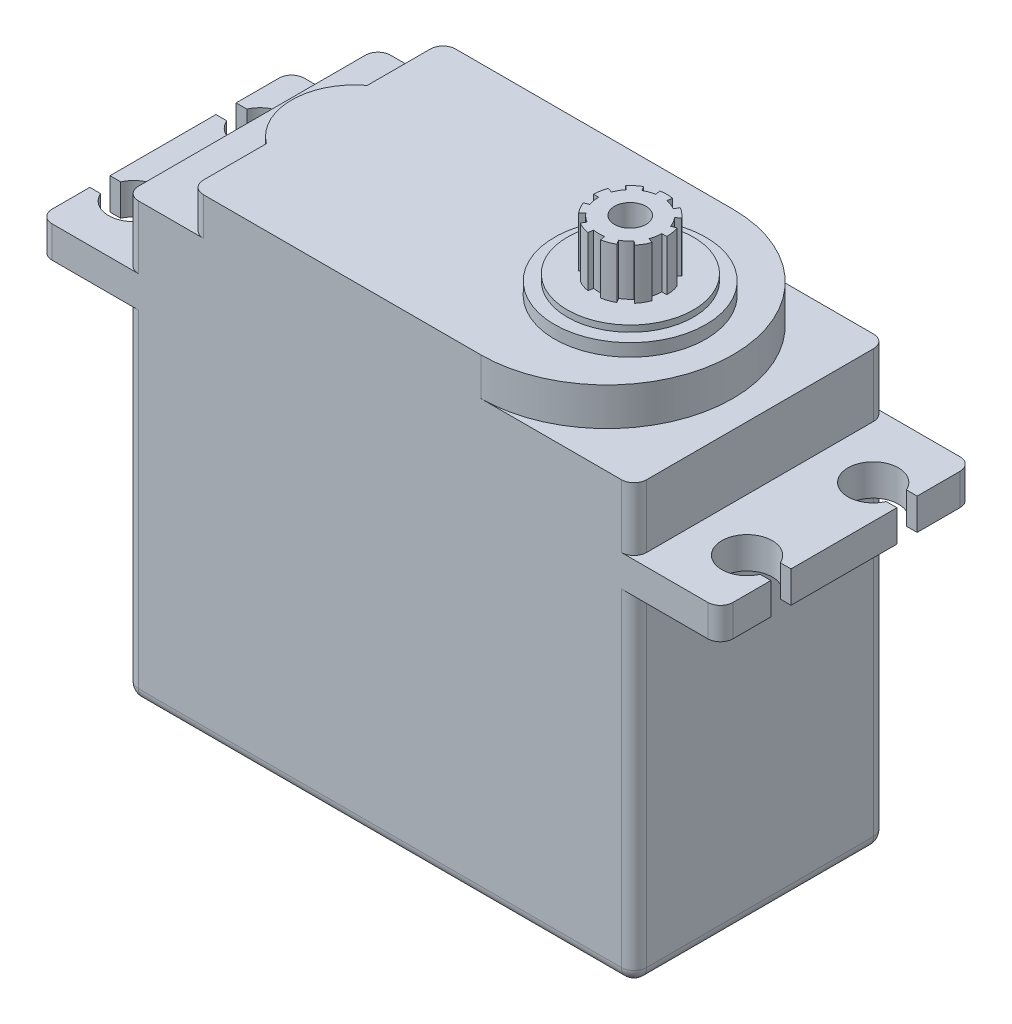
SolidWorks part; units mm, degrees
ref_plane "前视基准面" through (0, 0, 0) normal (0, 0, 1) x (1, 0, 0)
ref_plane "上视基准面" through (0, 0, 0) normal (0, 1, 0) x (1, 0, 0)
ref_plane "右视基准面" through (0, 0, 0) normal (1, 0, 0) x (0, 0, -1)
sketch "草图1" plane through (0, 0, 0) normal (0, 0, 1) x (1, 0, 0)
  line L0 (0, 0) -> (-50000, 0) construction
  line L1 (0, 0) -> (0, 50000) construction
  line L2 (20.15, 8) -> (27, 8)
  line L3 (-20.15, 18.5) -> (20.15, 18.5)
  line L4 (-20.15, 18.5) -> (-20.15, 10.5)
  line L5 (-20.15, -19) -> (20.15, -19)
  line L6 (20.15, 18.5) -> (20.15, 10.5)
  line L7 (-27, 10.5) -> (-20.15, 10.5)
  line L8 (-27, 10.5) -> (-27, 8)
  line L9 (-27, 8) -> (-20.15, 8)
  line L10 (27, 10.5) -> (27, 8)
  line L11 (20.15, 10.5) -> (27, 10.5)
  line L12 (20.15, 8) -> (20.15, -19)
  line L13 (-20.15, 8) -> (-20.15, -19)
  dimension "D1" = 8
  dimension "D2" = 6.85
  dimension "D3" = 2.5
  dimension "D4" = 40.3
  dimension "D5" = 27
  dimension "D6" = 54
  dimension "D7" = 20.15
extrude "凸台-拉伸1" add sketch "草图1" along normal blind 20
fillet "圆角1" radius 1 18 edges at (-20.15, 14.5, 20) (20.15, 14.5, 20) (20.15, 18.5, 10) (-20.15, 18.5, 10) (20.15, 14.5, 0) (-20.15, 14.5, 0) (-20.15, -19, 10) (0, -19, 20) (20.15, -19, 10) (0, -19, 0) (-20.15, -5.5, 0) (20.15, -5.5, 0) (20.15, -5.5, 20) (-20.15, -5.5, 20) (27, 9.25, 0) (27, 9.25, 20) (-27, 9.25, 0) (-27, 9.25, 20)
sketch "草图2" plane through (0, 10.5, 0) normal (0, 1, 0) x (1, 0, 0)
  line L0 (-0.1717, -10.2) -> (49999.8283, -10.2) construction
  line L1 (0, 0) -> (0, -50000) construction
  line L2 (-26.148, -4.4) -> (-29.2227, -4.4)
  line L3 (-24.315, -5.2) -> (-30.8838, -5.2) construction
  line L4 (-24, -15) -> (-30.5688, -15) construction
  line L5 (-29.2227, -4.4) -> (-29.2227, -6)
  line L6 (-26.148, -6) -> (-29.2227, -6)
  line L7 (-26.148, -14.4) -> (-29.2227, -14.4)
  line L8 (-29.2227, -16) -> (-29.2227, -14.4)
  line L9 (-26.148, -16) -> (-29.2227, -16)
  line L10 (26.148, -16) -> (29.2227, -16)
  line L11 (29.2227, -16) -> (29.2227, -14.4)
  line L12 (26.148, -14.4) -> (29.2227, -14.4)
  line L13 (29.2227, -4.4) -> (29.2227, -6)
  line L14 (26.148, -6) -> (29.2227, -6)
  line L15 (26.148, -4.4) -> (29.2227, -4.4)
  arc A0 (-26.148, -14.4) -> (-26.148, -16) centre (-24.315, -15.2) cw
  arc A1 (26.148, -14.4) -> (26.148, -16) centre (24.315, -15.2) ccw
  arc A2 (-26.148, -6) -> (-26.148, -4.4) centre (-24.315, -5.2) ccw
  arc A3 (26.148, -6) -> (26.148, -4.4) centre (24.315, -5.2) cw
  point P21 (-29.2227, -5.2)
  dimension "D2" = 10
  dimension "D1" = 48.63
  dimension "D3" = 2
extrude "切除-拉伸1" cut sketch "草图2" against normal blind 20
sketch "草图3" plane through (0, 18.5, 0) normal (0, 1, 0) x (1, 0, 0)
  line L0 (-40.2617, -10) -> (49959.7383, -10) construction
  line L1 (-14, 0) -> (8, 0)
  line L2 (-15, -1) -> (-15, -6)
  line L3 (-14, -20) -> (8, -20)
  line L4 (-15, -14) -> (-15, -19)
  line L5 (0, 0) -> (0, 50000) construction
  line L7 (-26.8677, 6.7729) -> (25, 6.7729)
  line L8 (-26.8677, 6.7729) -> (-26.8677, -28.4888)
  line L9 (-26.8677, -28.4888) -> (25, -28.4888)
  line L10 (25, 6.7729) -> (25, -28.4888)
  arc A0 (8, -20) -> (8, 0) centre (8, -10) ccw
  arc A1 (-15, -6) -> (-15, -14) centre (-12, -10) ccw
  arc A2 (-14, -20) -> (-15, -19) centre (-14, -19) cw
  arc A3 (-15, -1) -> (-14, 0) centre (-14, -1) cw
  dimension "D2" = 1
  dimension "D1" = 25
extrude "切除-拉伸2" cut sketch "草图3" against normal blind 3
sketch "草图4" plane through (0, 18.5, 0) normal (0, 1, 0) x (1, 0, 0)
  line L0 (27, -14.4) -> (27, -6) construction
  circle A0 centre (9.85, -10) radius 6
  dimension "D1" = 17.15
extrude "凸台-拉伸2" add sketch "草图4" along normal blind 1
sketch "草图5" plane through (0, 19.5, 0) normal (0, 1, 0) x (1, 0, 0)
  line L0 (27, -14.4) -> (27, -6) construction
  circle A0 centre (9.8513, -9.9876) radius 5
  point P2 (27, -10.2)
  dimension "D1" = 17.15
extrude "凸台-拉伸3" add sketch "草图5" along normal blind 0.5
sketch "草图6" plane through (0, 20, 0) normal (0, 1, 0) x (1, 0, 0)
  line L1 (10.2841, -7.538) -> (10.3536, -7.1441)
  line L3 (11.3, -7.4885) -> (11.1, -7.8349)
  line L5 (12.0715, -8.1359) -> (11.7651, -8.393)
  line L7 (12.5751, -9.0081) -> (12.1992, -9.1449)
  line L8 (6.95, -10) -> (7.35, -10)
  line L10 (7.5008, -9.1449) -> (7.1249, -9.0081)
  line L13 (8.6, -7.8349) -> (8.4, -7.4885)
  line L14 (7.9349, -8.393) -> (7.6285, -8.1359)
  line L15 (9.4159, -7.538) -> (9.3464, -7.1441)
  line L16 (9.4159, -12.462) -> (9.3464, -12.8559)
  line L19 (8.4, -12.5115) -> (8.6, -12.1651)
  line L20 (27, -14.4) -> (27, -6) construction
  line L21 (7.6285, -11.8641) -> (7.9349, -11.607)
  line L23 (7.1249, -10.9919) -> (7.5008, -10.8551)
  line L25 (12.1992, -10.8551) -> (12.5751, -10.9919)
  line L28 (11.1, -12.1651) -> (11.3, -12.5115)
  line L29 (10.2841, -12.462) -> (10.3536, -12.8559)
  line L30 (11.7651, -11.607) -> (12.0715, -11.8641)
  line L31 (12.35, -10) -> (12.75, -10)
  arc A0 (7.1249, -10.9919) -> (7.6285, -11.8641) centre (9.85, -10) ccw
  arc A1 (7.35, -10) -> (7.5008, -10.8551) centre (9.85, -10) ccw
  arc A2 (7.1249, -9.0081) -> (6.95, -10) centre (9.85, -10) ccw
  arc A3 (8.4, -7.4885) -> (7.6285, -8.1359) centre (9.85, -10) ccw
  arc A4 (10.3536, -7.1441) -> (9.3464, -7.1441) centre (9.85, -10) ccw
  arc A5 (12.0715, -8.1359) -> (11.3, -7.4885) centre (9.85, -10) ccw
  arc A6 (12.75, -10) -> (12.5751, -9.0081) centre (9.85, -10) ccw
  arc A7 (12.0715, -11.8641) -> (12.5751, -10.9919) centre (9.85, -10) ccw
  arc A8 (10.3536, -12.8559) -> (11.3, -12.5115) centre (9.85, -10) ccw
  arc A9 (8.4, -12.5115) -> (9.3464, -12.8559) centre (9.85, -10) ccw
  arc A10 (7.9349, -8.393) -> (7.5008, -9.1449) centre (9.85, -10) ccw
  arc A11 (9.4159, -7.538) -> (8.6, -7.8349) centre (9.85, -10) ccw
  arc A12 (11.1, -7.8349) -> (10.2841, -7.538) centre (9.85, -10) ccw
  arc A13 (12.1992, -9.1449) -> (11.7651, -8.393) centre (9.85, -10) ccw
  arc A14 (12.1992, -10.8551) -> (12.35, -10) centre (9.85, -10) ccw
  arc A15 (11.1, -12.1651) -> (11.7651, -11.607) centre (9.85, -10) ccw
  arc A16 (9.4159, -12.462) -> (10.2841, -12.462) centre (9.85, -10) ccw
  arc A17 (7.9349, -11.607) -> (8.6, -12.1651) centre (9.85, -10) ccw
  circle A18 centre (9.85, -10) radius 1
  dimension "D1" = 17.15
extrude "凸台-拉伸4" add sketch "草图6" along normal blind 4
hole_wizard "M3 螺纹孔1" positions "3D草图2" profile "草图8" tap size "M3" standard "GB"
sketch3d "3D草图2"
  line L0 (9.85, 24, 10) -> (9.85, 20, 10) construction
  point P0 (9.85, 24, 10)
sketch "草图8" plane through (9.85, 24, 10) normal (1, 0, 0) x (0, 0, 1)
  line L0 (0, 0) -> (0, 8.2511)
  line L1 (0, 8.2511) -> (1.25, 7.5)
  line L2 (1.25, 7.5) -> (1.25, 0)
  line L5 (1.25, 0) -> (0, 0)
  line L10 (0, 8.2511) -> (-1.25, 7.5) construction
  line L11 (0, -6.35) -> (0, 107.95) construction
  dimension "螺纹孔钻头直径" = 2.5
  dimension "螺纹孔钻头深度" = 7.5
  dimension "导头角度" = 118
cosmetic thread "孔螺蚊线1" parameters "D1"=6, "D2"=3
